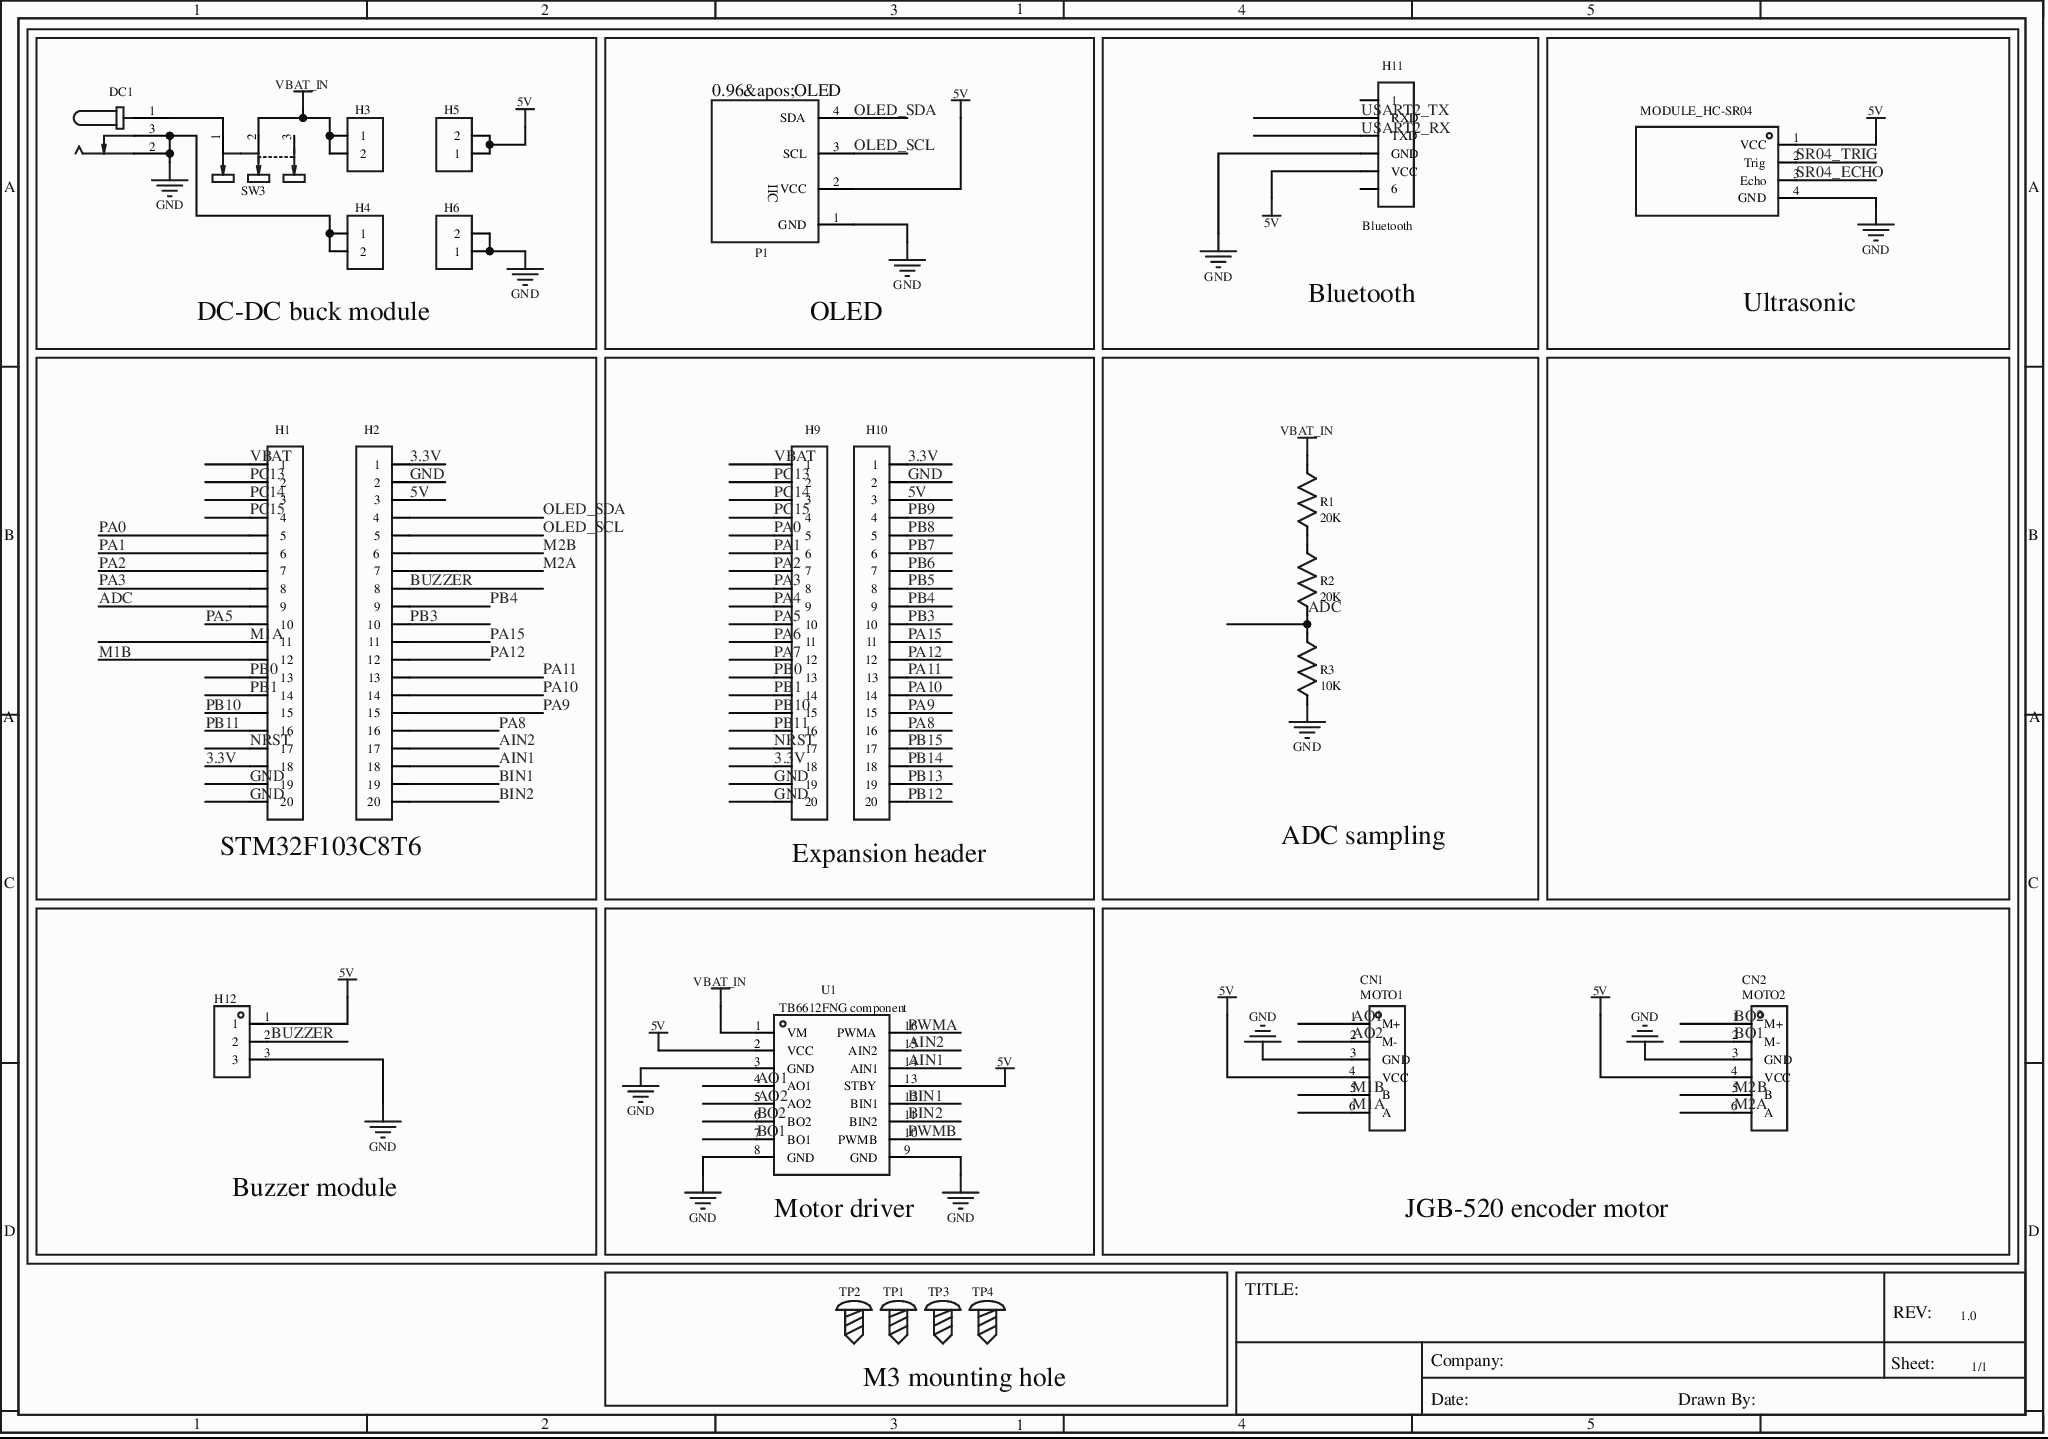
[diagram p0: MISC51780-3.schdoc]
# Altium project MISC51780-2.PrjPcb
1 sheet, 24 parts. Net scope: global (net labels, ports and power ports of the same name join across sheets).
Board file: MISC51780.pcbdoc

## Sheet MISC51780-3.schdoc
size 292 x 204 mm; Name: MISC51780; REV: 1.0; Sheet: 1/1; @Page No: 1; @Page Count: 1; @Schematic Name: MISC51780; @Project Name: MISC51780; @Board Name: MISC51780; @Update Date: 2025-03-20; @Create Time: 21:48:26; @Update Time: 21:48:33; @Create Date: 2025-03-20

### Parts
CN1  MOTO1  [CONN-TH_6P-P2.50_X8821WR-06S-N2SN]
CN2  MOTO2  [CONN-TH_6P-P2.50_X8821WR-06S-N2SN]
DC1  DC005_C431533  [DC-IN-TH_DC005]  (value not drawn)
H1  HDR-F-2.54_1x20  [HDR-F-2.54_1X20]  (value not drawn)
H2  HDR-F-2.54_1x20  [HDR-F-2.54_1X20]  (value not drawn)
H3  HDR-F-2.54_1x2  [HDR-F-2.54_1X2]  (value not drawn)
H4  HDR-F-2.54_1x2  [HDR-F-2.54_1X2]  (value not drawn)
H5  HDR-F-2.54_1x2  [HDR-F-2.54_1X2]  (value not drawn)
H6  HDR-F-2.54_1x2  [HDR-F-2.54_1X2]  (value not drawn)
H9  HDR-F-2.54_1x20  [HDR-F-2.54_1X20]  (value not drawn)
H10  HDR-F-2.54_1x20  [HDR-F-2.54_1X20]  (value not drawn)
H11  Bluetooth  [HDR-F-2.54_1X6]
H12  (no value)  [HDR-TH_3P-P2.54-V-F]
NO  MODULE_HC-SR04  [HC-SR04]
P1  0.96OLED_4P  [0.96OLED_4P]  (value not drawn)
R1  20K  [R0805]
R2  20K  [R0805]
R3  10K  [R0805]
SW3  SS-12D10L5  [SW-TH_SS-12D10L5]  (value not drawn)
TP1  M3 standoff with silkscreen  [M3铜柱]  (value not drawn)
TP2  M3 standoff with silkscreen  [M3铜柱]  (value not drawn)
TP3  M3 standoff with silkscreen  [M3铜柱]  (value not drawn)
TP4  M3 standoff with silkscreen  [M3铜柱]  (value not drawn)
U1  TB6612FNG component  [TB6612FNG封装]

### Blocks framed on the sheet
DC-DC buck module: DC1 H3-H6 SW3
OLED: P1
Bluetooth: H11
Ultrasonic: NO
STM32F103C8T6: H1 H2
Expansion header: H9 H10
ADC sampling: R1-R3
Buzzer module: H12
Motor driver: U1
JGB-520 encoder motor: CN1 CN2
M3 mounting hole: TP1-TP4

### Nets
5V: CN1.4(VCC) CN2.4(VCC) H2.3 H5.1 H5.2 H10.3 H11.5(VCC) H12.1 NO.1(VCC) P1.2(VCC) U1.2(VCC) U1.13(STBY)
GND: CN1.3(GND) CN2.3(GND) DC1.2 DC1.3 H1.19 H1.20 H2.2 H4.1 H4.2 H6.1 H6.2 H9.19 H9.20 H10.2 H11.4(GND) H12.3 NO.4(GND) P1.1(GND) R3.1 U1.3(GND) U1.8(GND) U1.9(GND)
VBAT_IN: H3.1 H3.2 R1.2 SW3.2 U1.1(VM)
3.3V: H1.18 H2.1 H9.18 H10.1
ADC: H1.9 H9.9 R2.1 R3.2  [also labelled PA4]
AIN1: H2.18 H10.18 U1.14(AIN1)  [also labelled PB14]
AIN2: H2.17 H10.17 U1.15(AIN2)  [also labelled PB15]
AO1: CN1.1(M+) U1.4(AO1)
AO2: CN1.2(M-) U1.5(AO2)
BIN1: H2.19 H10.19 U1.12(BIN1)  [also labelled PB13]
BIN2: H2.20 H10.20 U1.11(BIN2)  [also labelled PB12]
BO1: CN2.2(M-) U1.7(BO1)
BO2: CN2.1(M+) U1.6(BO2)
BUZZER: H2.8 H10.8 H12.2  [also labelled PB5]
M1A: CN1.6(A) H1.11 H9.11  [also labelled PA6]
M1B: CN1.5(B) H1.12 H9.12  [also labelled PA7]
M2A: CN2.6(A) H2.7 H10.7  [also labelled PB6]
M2B: CN2.5(B) H2.6 H10.6  [also labelled PB7]
NRST: H1.17 H9.17
OLED_SCL: H2.5 H10.5 P1.3(SCL)  [also labelled PB8]
OLED_SDA: H2.4 H10.4 P1.4(SDA)  [also labelled PB9]
PA0: H1.5 H9.5 NO.2(Trig)  [also labelled SR04_TRIG]
PA1: H1.6 H9.6 NO.3(Echo)  [also labelled SR04_ECHO]
PA2: H1.7 H9.7 H11.2(RXD)  [also labelled USART2_TX]
PA3: H1.8 H9.8 H11.3(TXD)  [also labelled USART2_RX]
PA5: H1.10 H9.10
PA8: H2.16 H10.16 U1.10(PWMB)  [also labelled PWMB]
PA9: H2.15 H10.15  [also labelled USART1_TX]
PA10: H2.14 H10.14  [also labelled USART1_RX]
PA11: H2.13 H10.13 U1.16(PWMA)  [also labelled PWMA]
PA12: H2.12 H10.12
PA15: H2.11 H10.11
PB0: H1.13 H9.13
PB1: H1.14 H9.14
PB3: H2.10 H10.10
PB4: H2.9 H10.9
PB10: H1.15 H9.15
PB11: H1.16 H9.16
PC13: H1.2 H9.2
PC14: H1.3 H9.3
PC15: H1.4 H9.4
VBAT: H1.1 H9.1
NetDC1_1: DC1.1 SW3.1
NetR1_1: R1.1 R2.2

Not connected (* = marked no-connect by the designer): H11 1* 6*; SW3 3*

### Notes on the sheet
- 1
- 2
- 3
- 4
- 5
- A
- B
- C
- D
- TITLE:
- Company:
- Sheet:
- REV:
- 1.0
- 1/1
- Date:
- Drawn By:

### Library data of the parts
CN1 = X8821WR-06S-N0SN: Manufacturer: XKB Enterprise; Convert to PCB: yes; Origin Footprint: CONN-TH_6P-P2.50_X8821WR-06S-N2SN; Device: X8821WR-06S-N0SN; Symbol: MOTO1; Add into BOM: yes; Supplier: LCSC; SupplierPart: C388743; ManufacturerPart: X8821WR-06S-N0SN; JLCPCB Part Class: Extended Part; FootprintName: CONN-TH_6P-P2.50_X8821WR-06S-N2SN
CN2 = X8821WR-06S-N0SN: Manufacturer: XKB Enterprise; Symbol: MOTO1; Convert to PCB: yes; Origin Footprint: CONN-TH_6P-P2.50_X8821WR-06S-N2SN; Device: X8821WR-06S-N0SN; Add into BOM: yes; Supplier: LCSC; SupplierPart: C388743; ManufacturerPart: X8821WR-06S-N0SN; JLCPCB Part Class: Extended Part; FootprintName: CONN-TH_6P-P2.50_X8821WR-06S-N2SN
DC1 = DC005: Manufacturer: SHOU HAN; Convert to PCB: yes; Origin Footprint: DC-IN-TH_DC005; Device: DC005; Symbol: DC005_C431533; Add into BOM: yes; Supplier: LCSC; SupplierPart: C431533; ManufacturerPart: DC005; JLCPCB Part Class: Extended Part; FootprintName: DC-IN-TH_DC005
H1 H2 H9 H10 = HDR-F-2.54_1x20: Convert to PCB: yes; Origin Footprint: HDR-F-2.54_1X20; Device: HDR-F-2.54_1x20; Symbol: HDR-F-2.54_1x20; Add into BOM: yes; SupplierPart: C50984; Supplier: LCSC; FootprintName: HDR-F-2.54_1X20
H3-H6 = HDR-F-2.54_1x2: Convert to PCB: yes; Origin Footprint: HDR-F-2.54_1X2; Device: HDR-F-2.54_1x2; Symbol: HDR-F-2.54_1x2; Add into BOM: yes; SupplierPart: C49661; Supplier: LCSC; FootprintName: HDR-F-2.54_1X2
H11 = Bluetooth: Convert to PCB: yes; Origin Footprint: HDR-F-2.54_1X6; Device: Bluetooth; Symbol: Bluetooth; Add into BOM: yes; SupplierPart: C40877; Supplier: LCSC; FootprintName: HDR-F-2.54_1X6
H12 = HDR-F_2.54_1x3P: Symbol: PM254V-11-03-H85; ConvertToPcb: yes; ModelId: f3b3cc5aae9641bf9e56fc160cef875b; ModelName: HDR2.54-F-LI-1X3P; ModelTransform: 299.9994,100,0,0,0,0,0,0,-118.11; Device: HDR-F_2.54_1x3P; AddInBom: yes; SupplierPart: C541850; Supplier Footprint: 插件; FootprintName: HDR-TH_3P-P2.54-V-F
NO = HC-SR04: Convert to PCB: yes; 美岩编码: M00001; 单价: 3.15; Origin Footprint: HC-SR04; Device: HC-SR04; Symbol: MODULE_HC-SR04; Add into BOM: yes; Manufacturer: -; ManufacturerPart: HC-SR04; Supplier: 欣薇电子; SupplierPart: -; FootprintName: HC-SR04
P1 = 0.96'OLED-IIC(4Pin): Convert to PCB: yes; Origin Footprint: 0.96OLED_4P; Device: 0.96'OLED-IIC(4Pin); Symbol: 0.96OLED_4P; Add into BOM: yes; ManufacturerPart: 0.96'OLED-IIC(4Pin); FootprintName: 0.96OLED_4P
R1 R2 = 20K: Convert to PCB: yes; Origin Footprint: R0805; Device: 20K; Symbol: 20K; Add into BOM: yes; FootprintName: R0805
R3 = 10K: Convert to PCB: yes; Origin Footprint: R0805; Device: 10K; Symbol: 10K; Add into BOM: yes; FootprintName: R0805
SW3 = SS-12D10L5: Manufacturer: XKB Enterprise; Convert to PCB: yes; Origin Footprint: SW-TH_SS-12D10L5; Device: SS-12D10L5; Symbol: SS-12D10L5; Add into BOM: yes; Supplier: LCSC; SupplierPart: C319012; ManufacturerPart: SS-12D10L5; JLCPCB Part Class: Extended Part; FootprintName: SW-TH_SS-12D10L5
TP1-TP4 = M3铜柱带丝印: Convert to PCB: yes; Origin Footprint: M3 standoff; Device: M3 standoff with silkscreen; Symbol: M3 standoff with silkscreen; Add into BOM: yes; FootprintName: M3 standoff
U1 = TB6612FNG-原件: Origin Footprint: TB6612FNG footprint; Convert to PCB: yes; Device: TB6612FNG component; Symbol: TB6612FNG component; Add into BOM: yes; FootprintName: TB6612FNG footprint